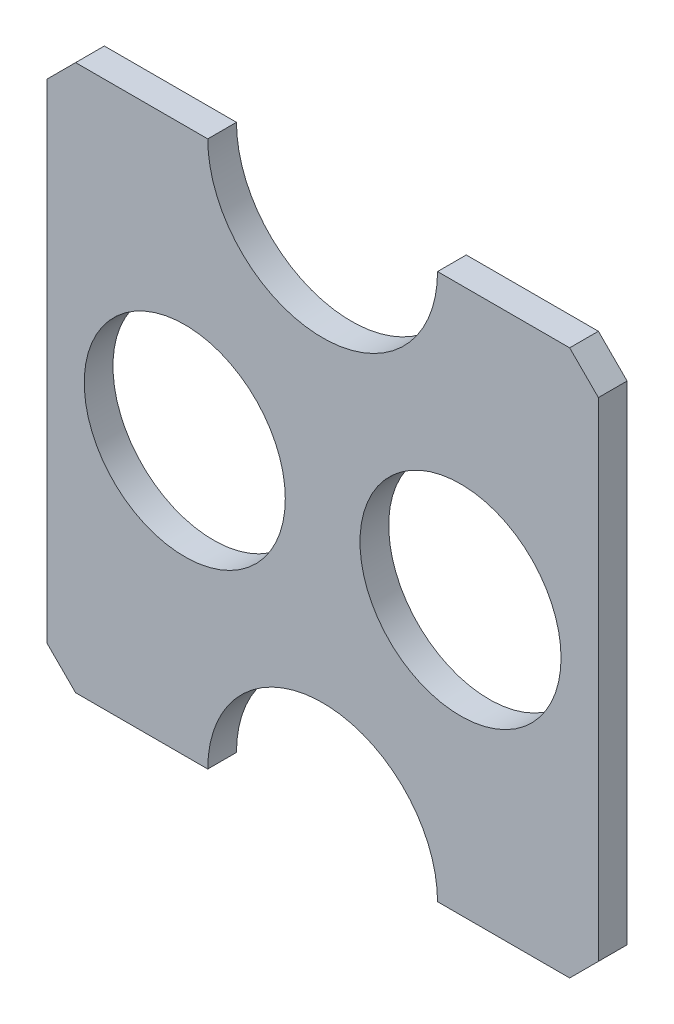
SolidWorks part; units mm, degrees
ref_plane "Front Plane" through (0, 0, 0) normal (0, 0, 1) x (1, 0, 0)
ref_plane "Top Plane" through (0, 0, 0) normal (0, 1, 0) x (1, 0, 0)
ref_plane "Right Plane" through (0, 0, 0) normal (1, 0, 0) x (0, 0, -1)
sketch "Sketch1" plane through (0, 0, 0) normal (0, 0, 1) x (1, 0, 0)
  line L0 (0, 95) -> (231.238, 95) construction
  line L1 (10, 0) -> (56, 0)
  line L2 (0, 10) -> (0, 180)
  line L3 (10, 190) -> (56, 190)
  line L4 (192, 10) -> (192, 180)
  line L5 (96, 190) -> (96, -60.6795) construction
  line L6 (182, 190) -> (192, 180)
  line L7 (0, 180) -> (10, 190)
  line L8 (48, 257.1072) -> (48, -37.0939) construction
  line L9 (144, 276.8244) -> (144, -53.179) construction
  line L10 (10, 0) -> (0, 10)
  line L11 (182, 0) -> (192, 10)
  line L12 (136, 190) -> (182, 190)
  line L13 (136, 0) -> (182, 0)
  arc A0 (56, 190) -> (136, 190) centre (96, 190) ccw
  arc A1 (136, 0) -> (56, 0) centre (96, 0) ccw
  circle A2 centre (48, 95) radius 35
  circle A3 centre (144, 95) radius 35
  point P0 (0, 0)
  point P1 (192, 190)
  point P2 (0, 190)
  point P3 (192, 0)
  dimension "D3" = 80
  dimension "D4" = 80
  dimension "D7" = 70
  dimension "D8" = 70
  dimension "D1" = 190
  dimension "D2" = 192
  dimension "D5" = 48
  dimension "D6" = 48
extrude "Boss-Extrude1" add sketch "Sketch1" along normal blind 10
